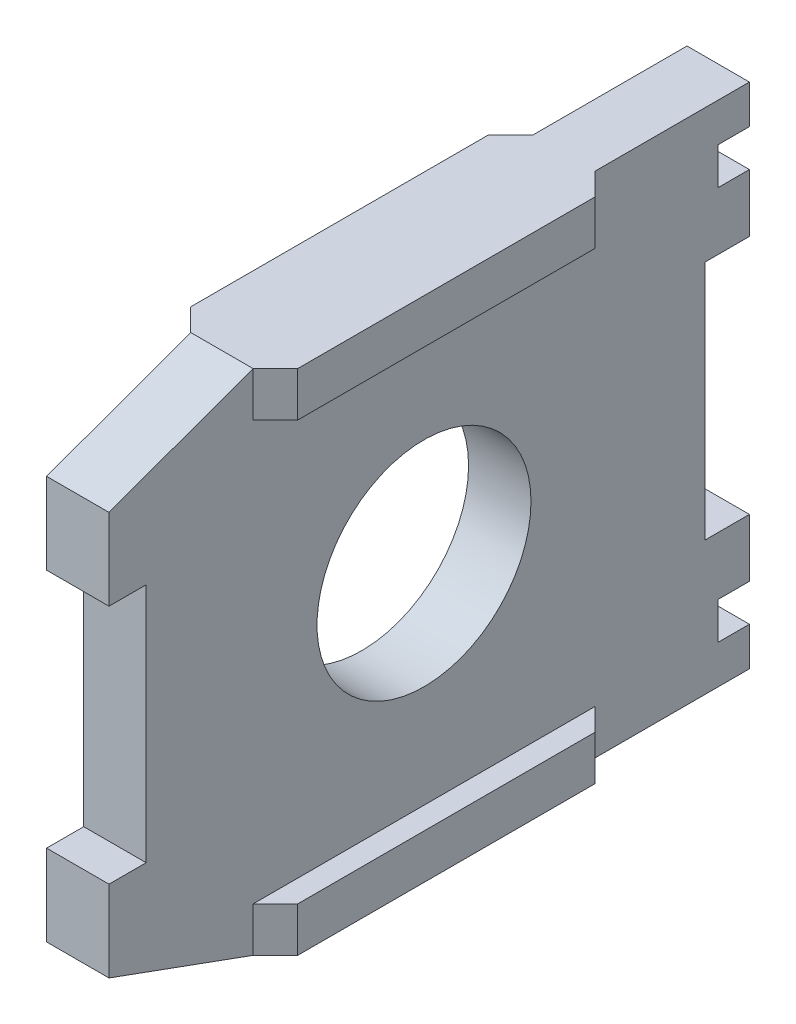
from build123d import *

# Parameters (mm, degrees)
EXTRUDE_1_DEPTH      = 2.1
EXTRUDE_1_DEPTH_BACK = 2.1
SKETCH_1_R           = 7.2
EXTRUDE_2_DEPTH      = 3
EXTRUDE_3_DEPTH      = 3


with BuildPart() as part:
    # 草图1 → 凸台-拉伸1 (new, two sides: drawn at the far end of the back side and taken through both)
    with BuildSketch(Plane(origin=(0, 0, 0), x_dir=(0, 0, -1), z_dir=(1, 0, 0)).offset(-EXTRUDE_1_DEPTH_BACK)):
        Polygon((-21.2, 8.1), (-18.7, 8.1), (-18.7, -8.1), (-21.2, -8.1), (-21.2, -13.569488728), (-11.5, -17.1), (21.9, -17.1), (21.9, -14.5), (19.8, -14.5), (19.8, -12), (21.9, -12), (21.9, -8.1), (18.9, -8.1), (18.9, 8.1), (21.9, 8.1), (21.9, 12), (19.8, 12), (19.8, 14.5), (21.9, 14.5), (21.9, 17.1), (-11.5, 17.1), (-21.2, 13.569488728), align=None)
        Circle(SKETCH_1_R, mode=Mode.SUBTRACT)
    extrude(amount=EXTRUDE_1_DEPTH + EXTRUDE_1_DEPTH_BACK)

    # 草图2 → 凸台-拉伸2 (add)
    with BuildSketch(Plane(origin=(0, 17.1, 0), x_dir=(1, 0, 0), z_dir=(0, 1, 0))):
        Polygon((-3.6, -10), (-2.1, -11.5), (2.1, -11.5), (3.6, -10), (3.6, 10), (2.1, 11.5), (-2.1, 11.5), (-3.6, 10), align=None)
    extrude(amount=-EXTRUDE_2_DEPTH)

    # 草图3 → 凸台-拉伸3 (add)
    with BuildSketch(Plane(origin=(0, -17.1, 0), x_dir=(1, 0, 0), z_dir=(0, 1, 0))):
        Polygon((-3.6, -10), (-2.1, -11.5), (2.1, -11.5), (3.6, -10), (3.6, 10), (2.1, 11.5), (-2.1, 11.5), (-3.6, 10), align=None)
    extrude(amount=EXTRUDE_3_DEPTH)


solid = part.part
